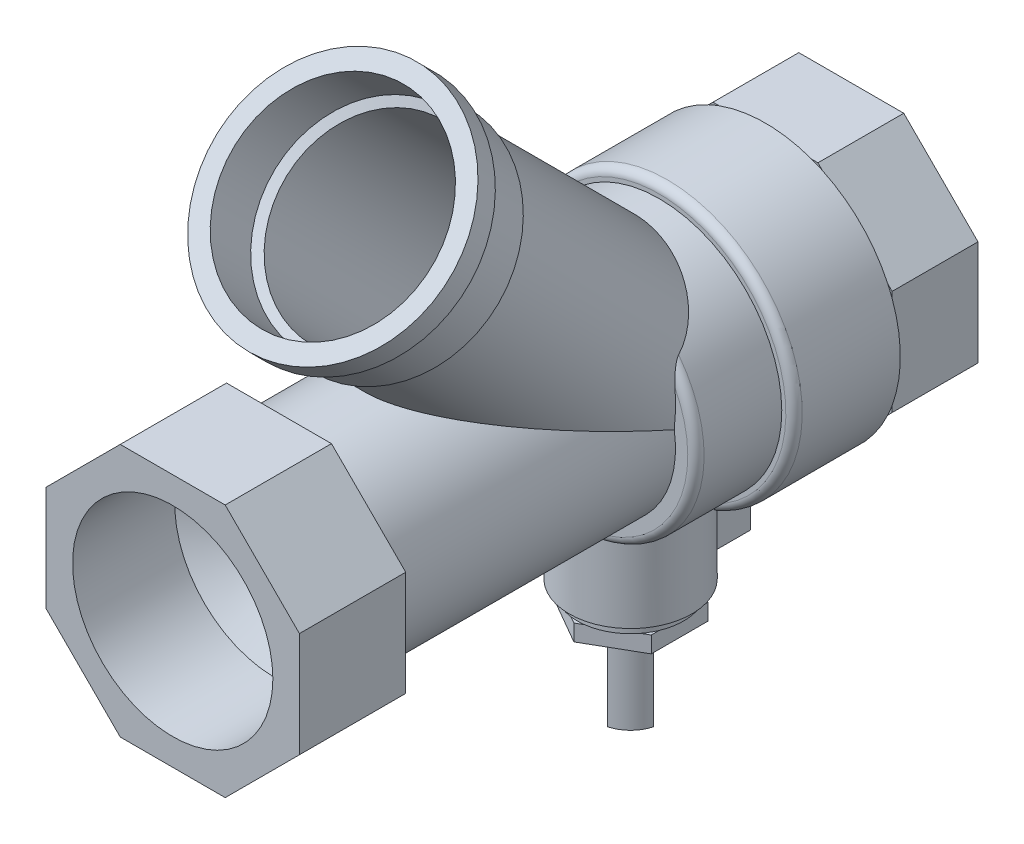
SolidWorks part; units mm, degrees
material "黄铜"
ref_plane "前视基准面" through (0, 0, 0) normal (0, 0, 1) x (1, 0, 0)
ref_plane "上视基准面" through (0, 0, 0) normal (0, 1, 0) x (1, 0, 0)
ref_plane "右视基准面" through (0, 0, 0) normal (1, 0, 0) x (0, 0, -1)
sketch "草图1" plane through (0, 0, 0) normal (0, 0, 1) x (1, 0, 0)
  circle A0 centre (0, 0) radius 15
  dimension "D1" = 30
extrude "凸台-拉伸1" add sketch "草图1" along normal blind 10.5
sketch "草图2" plane through (0, 0, 10.5) normal (0, 0, 1) x (1, 0, 0)
  circle A0 centre (0, 0) radius 12.5
  dimension "D1" = 25
extrude "凸台-拉伸2" add sketch "草图2" along normal blind 36
sketch "草图3" plane through (0, 0, 46.5) normal (0, 0, 1) x (1, 0, 0)
  line L0 (-1000, 0) -> (49000, 0) construction
  line L1 (6.4203, -15.5) -> (15.5, -6.4203)
  line L2 (15.5, -6.4203) -> (15.5, 6.4203)
  line L3 (15.5, 6.4203) -> (6.4203, 15.5)
  line L4 (6.4203, 15.5) -> (-6.4203, 15.5)
  line L5 (-6.4203, 15.5) -> (-15.5, 6.4203)
  line L6 (-15.5, 6.4203) -> (-15.5, -6.4203)
  line L7 (-15.5, -6.4203) -> (-6.4203, -15.5)
  line L8 (-6.4203, -15.5) -> (6.4203, -15.5)
  circle A0 centre (0, 0) radius 15.5 construction
  dimension "D1" = 31
extrude "凸台-拉伸3" add sketch "草图3" along normal blind 13
sketch "草图4" plane through (0, 0, 0) normal (0, 0, -1) x (-1, 0, 0)
  circle A0 centre (0, 0) radius 16.5
  dimension "D1" = 33
extrude "凸台-拉伸4" add sketch "草图4" along normal blind 13
sketch "草图6" plane through (0, 0, -13) normal (0, 0, -1) x (-1, 0, 0)
  line L0 (15.5, 6.4203) -> (15.5, -6.4203) construction
  line L1 (15.5, -6.4203) -> (15.5, 6.4203)
  line L2 (15.5, 6.4203) -> (6.4203, 15.5)
  line L3 (6.4203, 15.5) -> (-6.4203, 15.5)
  line L4 (-6.4203, 15.5) -> (-15.5, 6.4203)
  line L5 (-15.5, 6.4203) -> (-15.5, -6.4203)
  line L6 (-15.5, -6.4203) -> (-6.4203, -15.5)
  line L7 (-6.4203, -15.5) -> (6.4203, -15.5)
  line L8 (6.4203, -15.5) -> (15.5, -6.4203)
  circle A0 centre (0, 0) radius 15.5 construction
  dimension "D1" = 31
extrude "凸台-拉伸5" add sketch "草图6" along normal blind 10.5
fillet "圆角1" radius 1 2 edges at (15, 0, 10.5) (-16.5, 0, 0)
sketch "草图7" plane through (0, 0, 59.5) normal (0, 0, 1) x (1, 0, 0)
  circle A0 centre (0, 0) radius 5
  dimension "D1" = 10
hole_wizard "G3/4 螺纹孔1" positions "3D草图1" profile "草图8" tap size "G3/4" standard "GB"
sketch3d "3D草图1"
  point P0 (0, 0, 59.5)
sketch "草图8" plane through (0, 0, 59.5) normal (1, 0, 0) x (0, -1, 0)
  line L0 (0, 0) -> (0, 19.8605)
  line L1 (0, 19.8605) -> (12.25, 12.5)
  line L2 (12.25, 12.5) -> (12.25, 0)
  line L5 (12.25, 0) -> (0, 0)
  line L10 (0, 19.8605) -> (-12.25, 12.5) construction
  line L11 (0, -6.35) -> (0, 107.95) construction
  dimension "螺纹孔钻头直径" = 24.5
  dimension "螺纹孔钻头深度" = 12.5
  dimension "导头角度" = 118
cosmetic thread "孔螺蚊线1" parameters "D1"=12.5, "D2"=26.441
hole_wizard "G3/4 螺纹孔2" positions "草图9" profile "草图10" tap size "G3/4" standard "GB"
sketch "草图9" plane through (0, 0, -23.5) normal (0, 0, -1) x (-1, 0, 0)
  point P0 (0, 0)
sketch "草图10" plane through (0, 0, -23.5) normal (1, 0, 0) x (0, 1, 0)
  line L0 (0, 0) -> (0, 19.8605)
  line L1 (0, 19.8605) -> (12.25, 12.5)
  line L2 (12.25, 12.5) -> (12.25, 0)
  line L5 (12.25, 0) -> (0, 0)
  line L10 (0, 19.8605) -> (-12.25, 12.5) construction
  line L11 (0, -6.35) -> (0, 107.95) construction
  dimension "螺纹孔钻头直径" = 24.5
  dimension "螺纹孔钻头深度" = 12.5
  dimension "导头角度" = 118
cosmetic thread "孔螺蚊线2" parameters "D1"=12.5, "D2"=26.441
ref_plane "基准面1" through (0, -16.5, 0) normal (0, -1, 0) x (-1, 0, 0)
ref_plane "基准面2" through (0, -23.5, 0) normal (0, -1, 0) x (-1, 0, 0)
sketch "草图12" plane through (0, -23.5, 0) normal (0, -1, 0) x (-1, 0, 0)
  line L0 (0, -1000) -> (0, 49000) construction
  line L1 (6.4203, 23.5) -> (-6.4203, 23.5) construction
  line L2 (-1000.0119, -11) -> (48999.9881, -11) construction
  line L5 (-2.2, 9) -> (2.2, 9)
  line L9 (-2.2, 3.6701) -> (-2.2, 9)
  line L10 (2.2, 3.6701) -> (2.2, 9)
  arc A0 (-2.2, 3.6701) -> (2.2, 3.6701) centre (0, -3.5) ccw
  dimension "D2" = 15
  dimension "D1" = 27
  dimension "D3" = 20
  dimension "D4" = 4.4
extrude "凸台-拉伸6" add sketch "草图12" against normal up to next
sketch "草图13" plane through (0, -23.5, 0) normal (0, -1, 0) x (1, 0, 0)
  circle A0 centre (0, 3.5) radius 6.5
  arc A1 (2.2, -3.6701) -> (-2.2, -3.6701) centre (0, 3.5) ccw construction
  dimension "D1" = 1
extrude "凸台-拉伸7" add sketch "草图13" along normal blind 1.25
sketch "草图14" plane through (0, -24.75, 0) normal (0, -1, 0) x (1, 0, 0)
  line L0 (-1000, 3.5) -> (49000, 3.5) construction
  line L1 (6, 6.9641) -> (0, 10.4282)
  line L2 (0, 10.4282) -> (-6, 6.9641)
  line L3 (-6, 6.9641) -> (-6, 0.0359)
  line L4 (-6, 0.0359) -> (0, -3.4282)
  line L5 (0, -3.4282) -> (6, 0.0359)
  line L6 (6, 0.0359) -> (6, 6.9641)
  line L7 (0, -996.5) -> (0, 49003.5) construction
  circle A0 centre (0, 3.5) radius 6 construction
  dimension "D1" = 12
extrude "凸台-拉伸8" add sketch "草图14" along normal blind 2
sketch "草图15" plane through (0, -26.75, 0) normal (0, -1, 0) x (1, 0, 0)
  circle A0 centre (0, 3.5) radius 4
  dimension "D1" = 8
extrude "凸台-拉伸9" add sketch "草图15" along normal blind 10
sketch "草图16" plane through (0, 0, 0) normal (1, 0, 0) x (0, 0, -1)
  line L0 (-1000, 0) -> (49000, 0) construction
  line L1 (2.1307, -12.5) -> (-35.1181, 24.7487)
  line L3 (-1029.0756, -12.5) -> (48970.9244, -12.5) construction
  line L5 (-46.5, -12.5) -> (-11, -12.5) construction
  line L6 (-10.3693, 9.8405) -> (-10.3693, -9.8405) construction
  point P15 (-10.3693, 0)
  dimension "D1" = 45
  dimension "D2" = 35
ref_plane "基准面3" through (0, -5.1847, 5.1847) normal (0, 0.7071, -0.7071) x (0, 0.7071, 0.7071)
sketch "草图17" plane through (0, -5.1847, 5.1847) normal (0, 0.7071, -0.7071) x (0, 0.7071, 0.7071)
  line L0 (7.5595, 16.7589) -> (7.5595, -16.7589)
  line L3 (-10.3455, 0) -> (42.3322, 0) construction
  line L4 (142128.463, -0.0175) -> (-176069.5885, 0.0216) construction
  point P1 (7.5595, 0)
ref_plane "基准面5" through (0, 5.3454, 5.3454) normal (0, -0.7071, -0.7071) x (-1, 0, 0)
sketch "草图18" plane through (0, 5.3454, 5.3454) normal (0, -0.7071, -0.7071) x (-1, 0, 0)
  line L0 (0, -1000) -> (0, 49000) construction
  circle A0 centre (0, -4.117) radius 12.5
  spline S0 degree 3 poles (-2.6926, -16.056) (-2.2667, -16.2382) (-1.8291, -16.3777) (-1.1548, -16.5199) (-0.927, -16.5561) (-0.4651, -16.6047) (-0.2322, -16.617) (0.4596, -16.6171) (0.9164, -16.5694) (1.5953, -16.4274) (1.821, -16.368) (2.2627, -16.2279) (2.4795, -16.1471) (2.6926, -16.056) knots 0 0 0 0 0.25 0.25 0.375 0.375 0.5 0.5 0.75 0.75 0.875 0.875 1 1 1 1 construction
  dimension "D1" = 25
sweep "扫描2" add profiles "草图18" path "草图16"
sketch "草图19" plane through (0, 29.9334, 29.9334) normal (0, 0.7071, 0.7071) x (1, 0, 0)
  circle A0 centre (0, -4.117) radius 13.25
  dimension "D1" = 26.5
extrude "凸台-拉伸10" add sketch "草图19" along normal blind 7
sketch "草图20" plane through (0, 34.8831, 34.8831) normal (0, 0.7071, 0.7071) x (1, 0, 0)
  circle A0 centre (0, -4.117) radius 14.5
  dimension "D1" = 29
extrude "凸台-拉伸11" add sketch "草图20" along normal blind 3
hole_wizard "G3/4 螺纹孔3" positions "3D草图2" profile "草图23" tap size "G3/4" standard "GB"
sketch3d "3D草图2"
  line L0 (0, 34.0933, 39.9156) -> (0, 31.972, 37.7943) construction
  point P0 (0, 34.0933, 39.9156)
sketch "草图23" plane through (0, 34.0933, 39.9156) normal (1, 0, 0) x (0, -0.7071, 0.7071)
  line L0 (0, 0) -> (0, 14.3605)
  line L1 (0, 14.3605) -> (12.25, 7)
  line L2 (12.25, 7) -> (12.25, 0)
  line L5 (12.25, 0) -> (0, 0)
  line L10 (0, 14.3605) -> (-12.25, 7) construction
  line L11 (0, -6.35) -> (0, 107.95) construction
  dimension "螺纹孔钻头直径" = 24.5
  dimension "螺纹孔钻头深度" = 7
  dimension "导头角度" = 118
cosmetic thread "孔螺蚊线3" parameters "D1"=7, "D2"=26.441
sketch "草图24" plane through (0, 37.0045, 37.0045) normal (0, 0.7071, 0.7071) x (1, 0, 0)
  circle A0 centre (0, -4.117) radius 11.25
  dimension "D1" = 22.5
extrude "切除-拉伸2" cut sketch "草图24" against normal blind 45
sketch "草图11" plane through (0, 0, -23.5) normal (0, 0, -1) x (-1, 0, 0)
  circle A0 centre (0, 0) radius 7.5
  dimension "D1" = 15
extrude "切除-拉伸1" cut sketch "草图11" against normal up to next
sketch "草图25" plane through (0, -36.75, 0) normal (0, -1, 0) x (1, 0, 0)
  line L0 (-1000, 3.5) -> (49000, 3.5) construction
  line L1 (0, 3.5) -> (35355.3391, 35358.8391) construction
  line L2 (1.0353, 7.3637) -> (-3.8637, 2.4647)
  line L3 (3.8637, 4.5353) -> (-1.0353, -0.3637)
  arc A0 (-1.0353, -0.3637) -> (3.8637, 4.5353) centre (0, 3.5) ccw
  circle A1 centre (0, 3.5) radius 4
  arc A2 (1.0353, 7.3637) -> (-3.8637, 2.4647) centre (0, 3.5) ccw
  dimension "D2" = 45
  dimension "D3" = 4
  dimension "D1" = 0
extrude "切除-拉伸3" cut sketch "草图25" against normal up to surface (10 mm away) up to face at (4, -26.75, 3.5)
